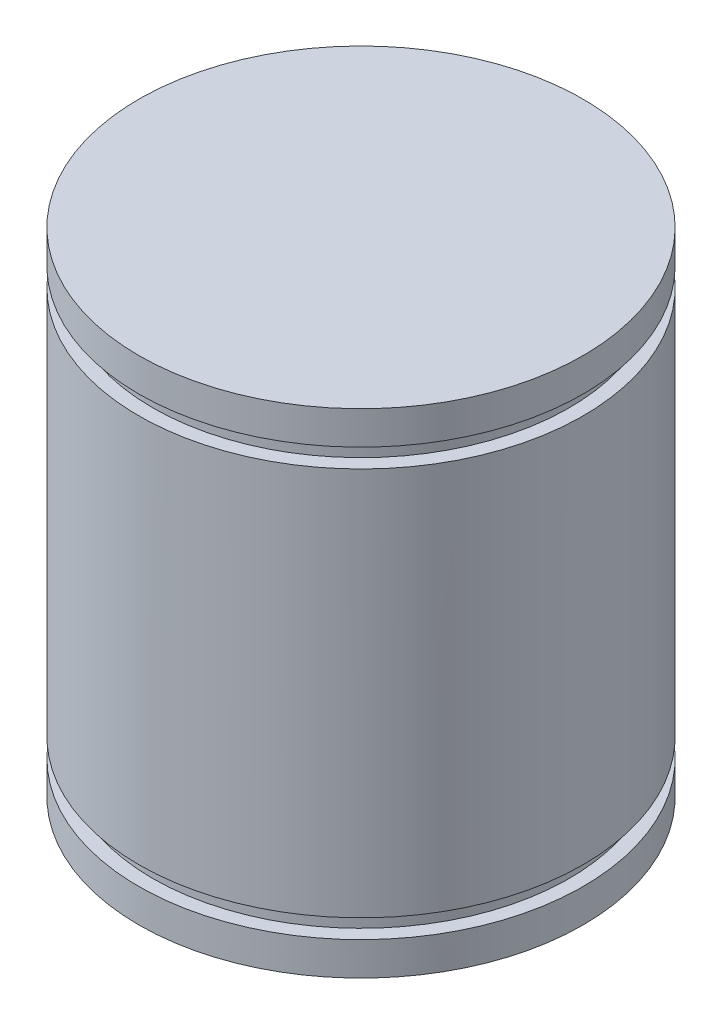
SolidWorks part; units mm, degrees
material "合金钢"
ref_plane "前视基准面" through (0, 0, 0) normal (0, 0, 1) x (1, 0, 0)
ref_plane "上视基准面" through (0, 0, 0) normal (0, 1, 0) x (1, 0, 0)
ref_plane "右视基准面" through (0, 0, 0) normal (1, 0, 0) x (0, 0, -1)
sketch "草图1" plane through (0, 0, 0) normal (0, 1, 0) x (1, 0, 0)
  circle A0 centre (0, 0) radius 20
  dimension "D1" = 40
extrude "凸台-拉伸1" add sketch "草图1" along normal blind 44.4
sketch "草图2" plane through (0, 0, 0) normal (0, 0, 1) x (1, 0, 0)
  line L0 (-20, 0) -> (20, 0) construction
  line L1 (-21.2896, 3) -> (-18.75, 3)
  line L2 (-21.2896, 3) -> (-21.2896, 4.7)
  line L3 (-21.2896, 4.7) -> (-18.75, 4.7)
  line L4 (-18.75, 3) -> (-18.75, 4.7)
  dimension "D1" = 3
  dimension "D2" = 1.7
  dimension "D3" = 18.75
revolve "切除-旋转1" cut sketch "草图2" angle 360 about axis through (0, 44.4, 0) along (0, -1, 0)
ref_plane "基准面1" through (0, 22.2, 0) normal (0, -1, 0) x (-1, 0, 0)
mirror "镜向1" about plane through (0, 22.2, 0) normal (0, -1, 0) of "切除-旋转1"
